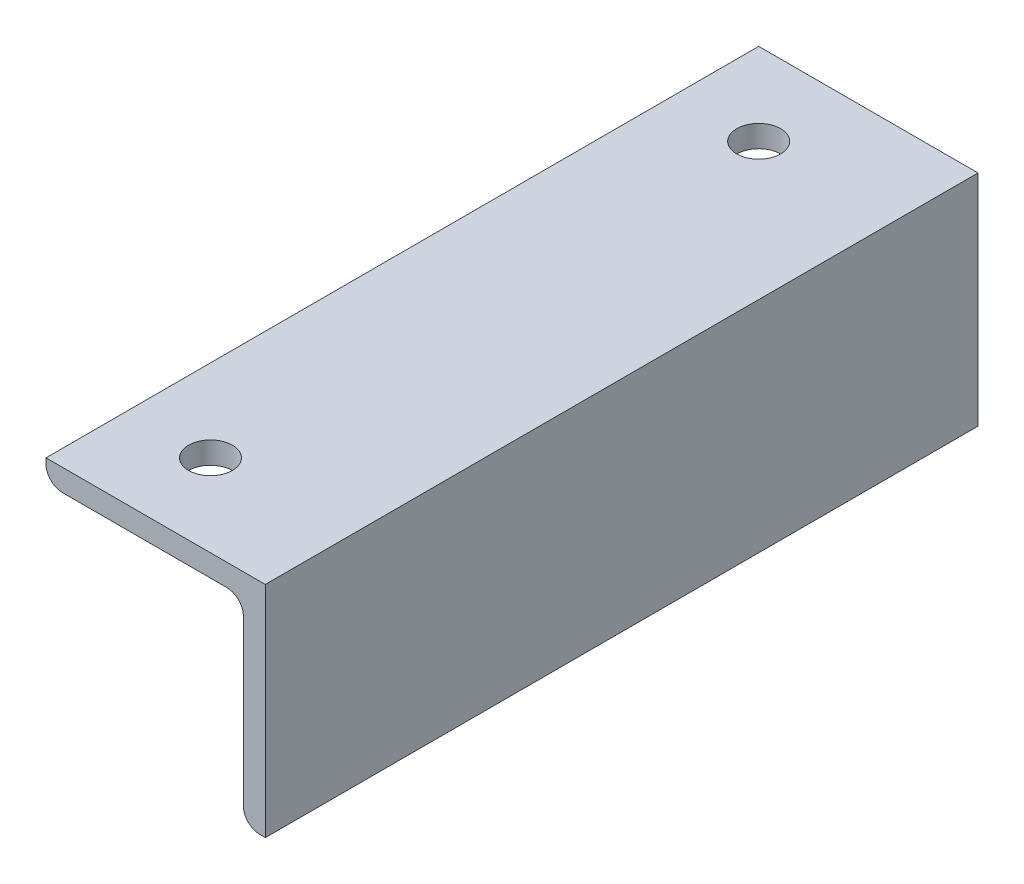
from build123d import *

# Parameters (mm, degrees)
BOSS_EXTRUDE1_DEPTH = 130
FILLET1_R           = 3
SKETCH2_R           = 4
CUT_EXTRUDE1_DEPTH  = 130


with BuildPart() as part:
    # Sketch1 → Boss-Extrude1 (new body)
    with BuildSketch(Plane.XY):
        Polygon((0, 0), (40, 0), (40, -40), (36, -40), (36, -4), (0, -4), align=None)
    extrude(amount=BOSS_EXTRUDE1_DEPTH)

    # Fillet1
    fillet1_edges = [part.edges().sort_by_distance(p)[0] for p in [
        (0, -4, 65),
        (36, -4, 65),
        (36, -40, 65),
    ]]
    fillet(fillet1_edges, radius=FILLET1_R)

    # Sketch2 → Cut-Extrude1 (cut)
    with BuildSketch(Plane.XZ.offset(4)):
        with Locations(Location((15, 115, 0), (0, 0, 270))):
            Circle(SKETCH2_R)
        with Locations(Location((15, 15, 0), (0, 0, 270))):
            Circle(SKETCH2_R)
    extrude(amount=-CUT_EXTRUDE1_DEPTH, mode=Mode.SUBTRACT)


solid = part.part
